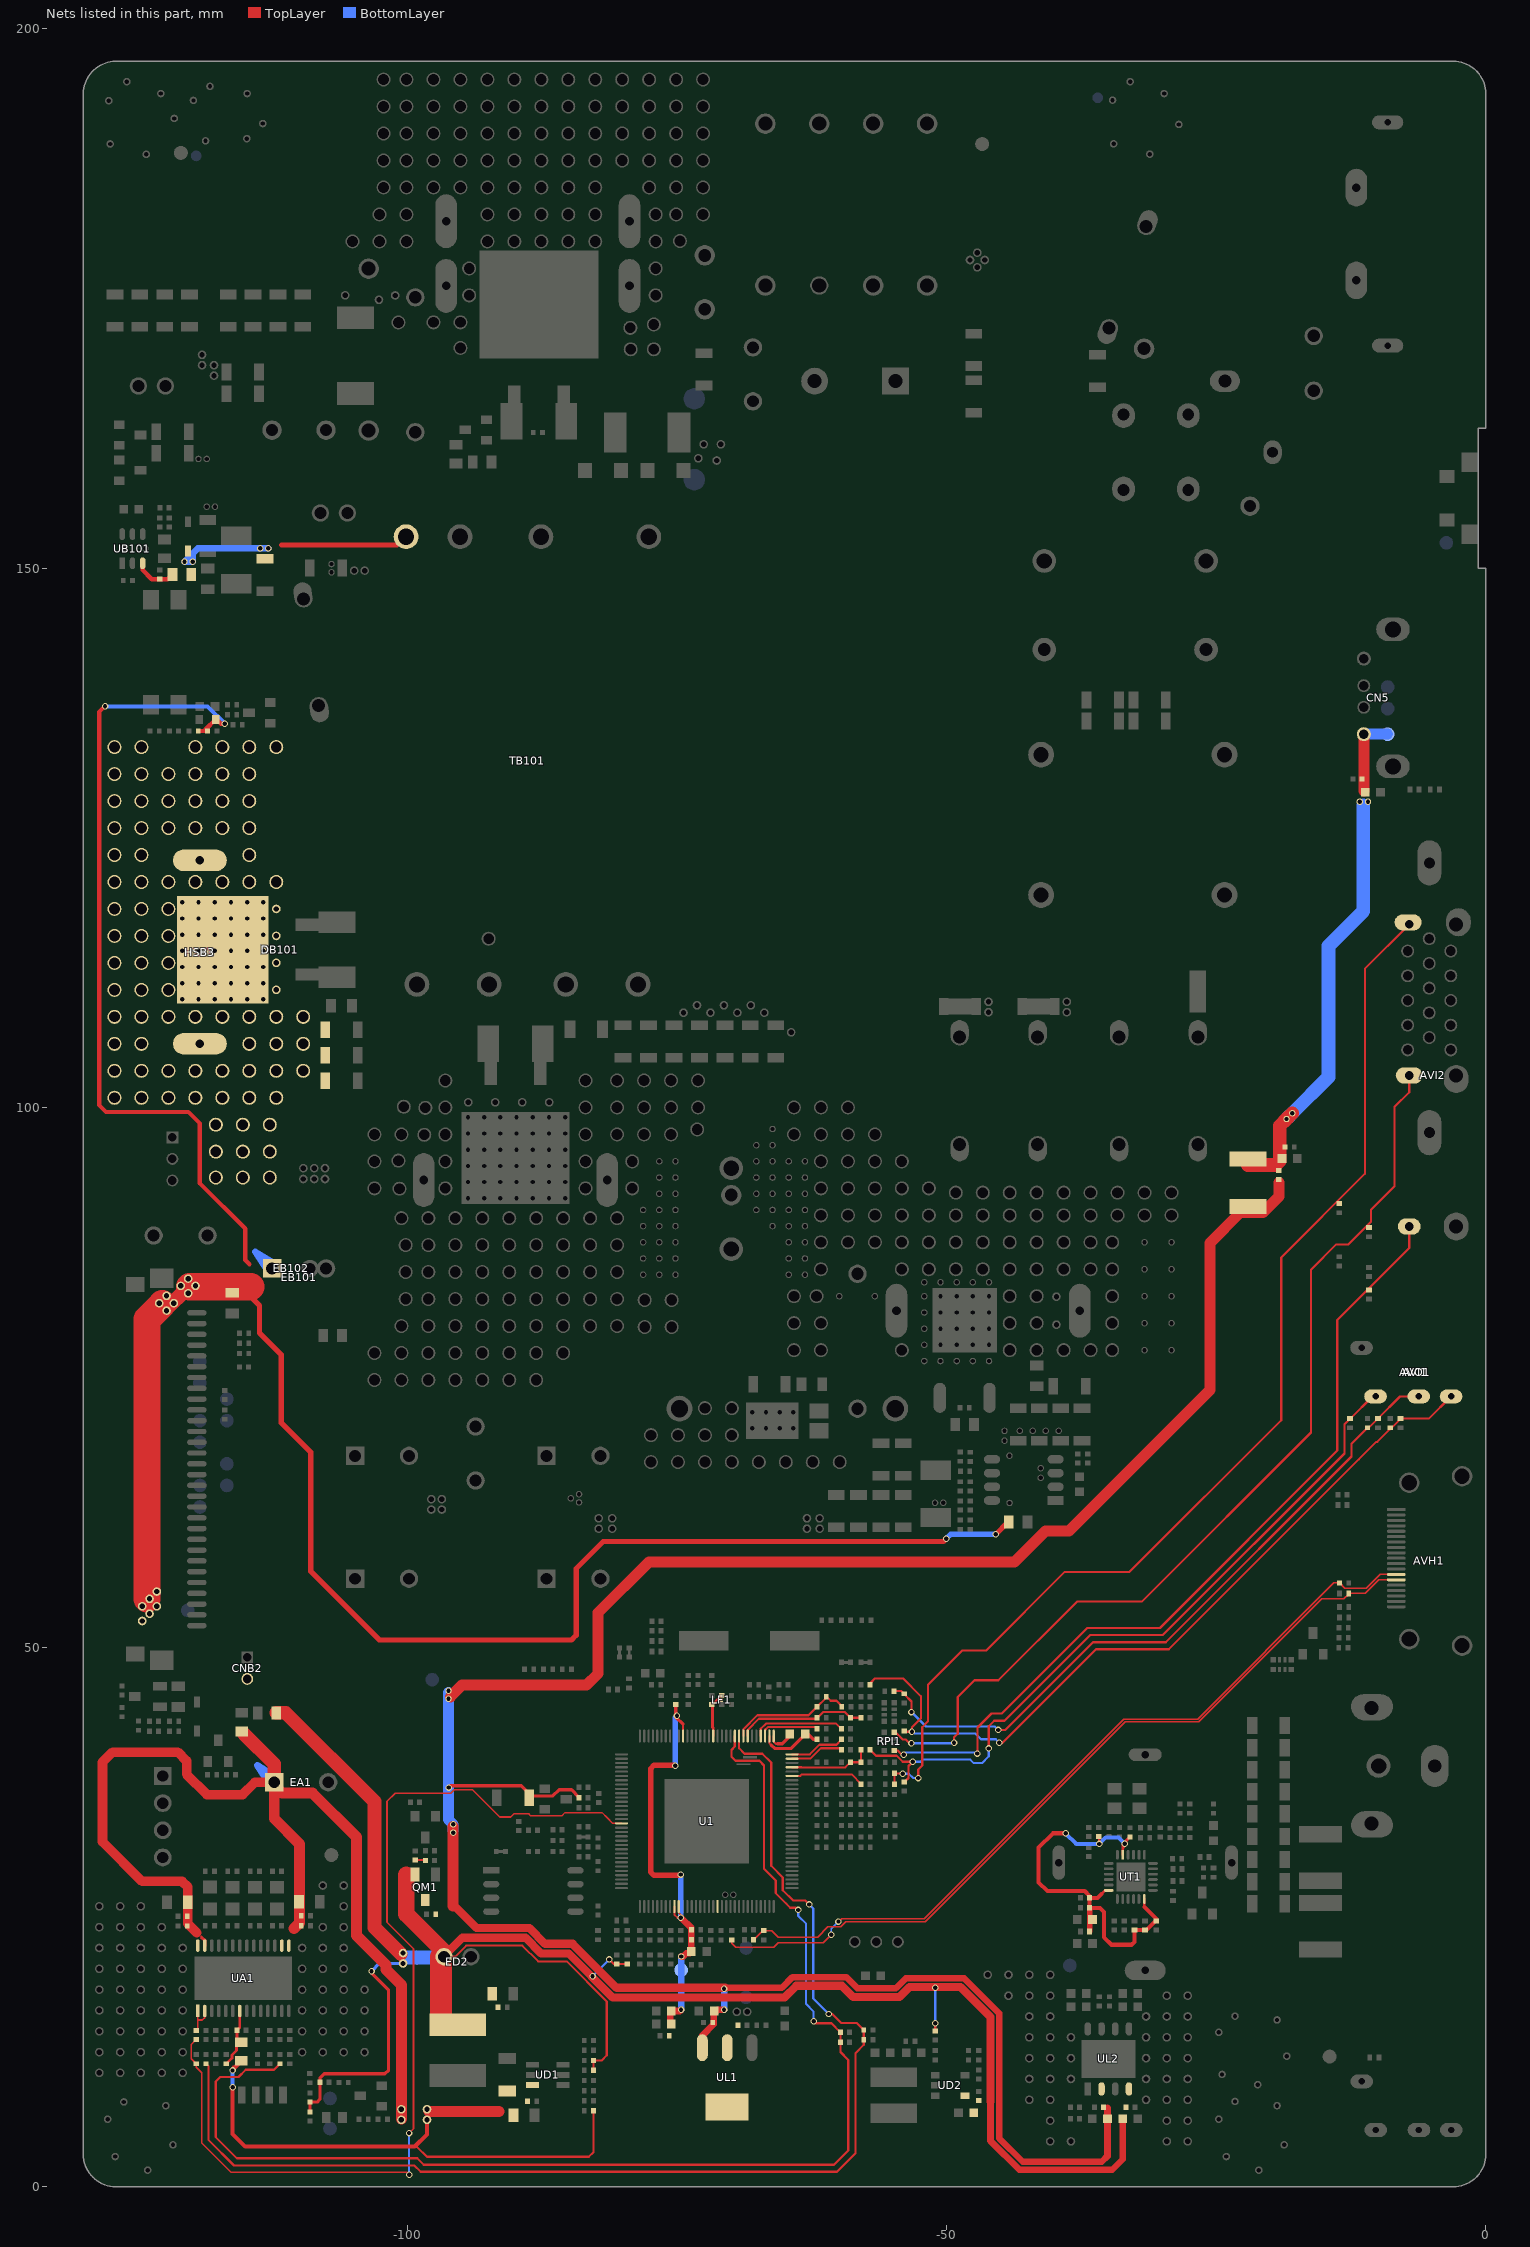
[diagram p0: the nets of this part, all layers, seen from the top]
# Altium PCB MISC84438.PcbDoc (part 7 of 15)
Units mm, origin at the board's own origin, x right, y up, seen from the top; angles counter-clockwise.
Board outline 130 x 197 mm, 2 copper layers (TopLayer, BottomLayer), stack 1.571 mm thick; 574 components, 314 nets, 2636 pads, 811 vias.

## Via types
v1: diameter 0.6, hole 0.4, TopLayer to BottomLayer, tented both sides, 780 vias
v2: diameter 0.7, hole 0.5, TopLayer to BottomLayer, tented both sides, 15 vias
v3: diameter 0.8, hole 0.6, TopLayer to BottomLayer, tented both sides, 12 vias
v4: diameter 0.8, hole 0.5, TopLayer to BottomLayer, tented both sides, 4 vias

## Nets (pads, with @x,y where several pads share a name; then routed paths per layer and width w, separated by ;. In a path a pad name is that pad's centre, name@x,y a point inside that pad or via, vN(x,y) a via of type N, cw(c..) or ccw(c..) an arc to the next point about the centre after c; other vN are vias at no path point) (continued)
3V3_Tun: CT5.2 CT6.1 CT9.1 CT18.2 CT27.1 LT1.1 LT2.2 LT12.2 RT18.1 UT1.11 UT1.18 UT1.24 | length 39
  TopLayer w0.203: RT18.1@-35.89,32.443 -35.839,32.392 v1(-35.839,31.763) ; UT1.11@-33.656,30.764 -33.656,31.407 -33.617,31.445
  TopLayer w0.229: -35.631,27.122 -35.29,27.464 UT1.18@-34.956,27.464 ; UT1.24@-31.656,26.664 -31.656,25.915 -31.648,25.908
  TopLayer w0.305: -33.617,31.445 -33.617,31.782 v1@-33.477,31.921 ; v1(-33.477,31.788) v1@-33.477,31.921 ; CT27.1@-32.982,32.417 v1@-33.477,31.921
  TopLayer w0.381: v1(-38.951,32.753) -40.132,32.753 -41.453,31.432 -41.453,28.194 -40.648,27.389 -37.179,27.389 -36.735,26.945 CT18.2@-36.735,26.772 ; -35.631,27.122 -35.982,26.772 CT18.2@-36.735,26.772 ; -31.648,25.908 -30.543,24.803 CT9.1@-30.543,24.631 -30.618,24.631 -31.468,23.781 LT1.1@-31.61,23.781 LT2.2@-32.575,23.781 -32.575,22.693 -32.848,22.42 -34.689,22.42 -35.382,23.114 -35.382,25.451 -35.776,25.844 CT5.2@-36.735,25.844 CT18.2@-36.735,26.772
  TopLayer w0.508: LT12.2@-36.735,23.66 CT5.2@-36.735,25.844
  BottomLayer w0.381: v1(-38.951,32.753) -37.96,31.763 v1(-35.839,31.763) -35.235,32.367 -34.057,32.367 v1(-33.477,31.788)
5V_M: CL1.2 CL2.2 CL6.2 CL7.2 CM2.1 F1.2 F2.1 pad.VIA5@-95.72,32.817 pad.VIA5@-95.72,33.579 pad.VIA5@-96.152,45.212 pad.VIA5@-96.152,45.974 QM1.D RO2.2 RO6.1 UL1.3 UL2.2 | length 232.1
  TopLayer w0.305: v1(-96.139,36.995) -95.987,37.147 -89.42,37.147 -88.493,36.22 -88.484,36.211 -86.471,36.211 -85.903,36.779 -84.75,36.779 -84.067,36.096 RO6.1@-84.067,36.065
  TopLayer w0.61: UL1.3@-72.623,12.877 -72.623,14.016 -71.577,15.062 -71.577,15.215 -71.577,16.002 -71.415,16.165 -71.183,16.396 v1(-70.612,16.396) ; v1@-70.51,18.433 -65.25,18.433 -64.255,19.428 -59.285,19.428 -58.253,18.396 -54.677,18.396 -53.75,19.323 -48.362,19.323 -45.098,16.058 -45.098,4.47 -42.926,2.299 -35.598,2.299 -35.07,2.827 CL7.2@-35.07,6.299 -35.07,7.29
  TopLayer w0.762: -95.606,26.01 -93.561,23.965 -88.648,23.965 -87.192,22.509 -84.64,22.509 -80.563,18.433 -70.612,18.433 v1@-70.51,18.433
  TopLayer w1.016: pad.VIA5@-95.987,45.402 -95.784,45.606 -94.907,46.482 -83.347,46.482 -82.283,47.546 -82.283,53.197 -77.568,57.912 -43.69,57.912 -40.819,60.782 -38.633,60.782 -25.578,73.838 -25.578,87.483 -22.76,90.301 -22.041,90.301 -20.66,90.301 -19.184,91.777 -19.184,93.098 ; -95.72,26.01 pad.VIA5@-95.72,32.817 pad.VIA5@-95.72,33.393
  BottomLayer w0.61: v1(-70.612,16.396) v1(-70.612,18.351)
  BottomLayer w1.016: pad.VIA5@-96.152,45.796 pad.VIA5@-96.152,45.212 -96.152,36.995 -96.152,34.011 pad.VIA5@-95.72,33.579 pad.VIA5@-95.72,33.033
5V_STB: 5V_STB.1 CD11.2 CD12.1 CD20.1 CD21.1 CD22.1 CL8.2 CL9.2 CM1.1 ED2.1 LD3.2 pad.VIA5@-100.368,20.688 pad.VIA5@-100.368,21.653 QM1.S R5V.1 RD8.1 RD13.2 RF8.2 RF9.2 RK1.2 RK13.1 RK15.1 RM1.2 UD2.4 UL2.4 | length 188.3
  TopLayer w0.203: RM1.2@-99.238,30.265 -98.323,30.265 CM1.1@-98.291,30.233 ; ED2.1@-96.846,21.311 ED2.1@-96.576,21.311 -95.53,21.311 -94.502,22.339 -89.306,22.339 -87.846,20.879 -85.204,20.879 -81.483,17.158 -81.483,12.167 -81.953,11.697 CD20.1@-82.721,11.697 RD13.2@-82.721,10.771 ; v1(-81.255,21.057) -80.827,20.629 RF8.2@-80.543,20.629 RF9.2@-79.578,20.629 ; RD8.1@-51.027,14.433 v1(-51.029,15.151)
  TopLayer w0.305: RK15.1@-108.991,6.927 RK13.1@-108.991,7.843 -108.324,7.843 -108.07,8.097 RK1.2@-108.07,9.677 -108.07,10.065 -107.675,10.461 -102.045,10.461 -101.711,10.795 -101.711,18.203 -103.289,19.781 v1(-103.289,19.977)
  TopLayer w0.61: -45.91,7.899 -45.91,4.242 -43.231,1.562 -34.633,1.562 -33.663,2.532 CL8.2@-33.663,6.299
  TopLayer w0.762: ED2.1@-96.139,21.806 -94.869,23.076 -89.016,23.076 -87.561,21.62 -85.008,21.62 -80.932,17.544 -64.99,17.544 -63.918,18.615 -59.673,18.615 -58.641,17.583 -54.341,17.583 -53.414,18.51 -48.699,18.51 -45.91,15.722 -45.91,7.899
  TopLayer w1.27: R5V.1@-112.113,43.917 -111.24,43.917 -103.022,35.699 -103.022,24.017 pad.VIA5@-100.568,21.562
  TopLayer w1.524: -100.051,28.905 -100.051,25.248 ED2.1@-96.576,21.773
  TopLayer w2.032: LD3.2@-96.846,15.164 ED2.1@-96.846,21.311
  BottomLayer w0.203: v1(-82.804,19.507) v1(-81.255,21.057) ; v1(-51.029,15.151) v1(-51.029,18.44)
  BottomLayer w0.305: v1(-103.289,19.977) -102.578,20.688 pad.VIA5@-100.368,20.688
  BottomLayer w1.27: -100.127,21.234 5V_STB.1@-99.085,21.234 -97.092,21.234 ED2.1@-96.576,21.234
5V_USB: CN5.1@-11.31,134.63 CU1.2 CU2.1 CU3.1 CU4.2 F1.1 F2.2 pad.VIA5@-10.922,128.372 pad.VIA5@-11.684,128.372 pad.VIA5@-17.936,99.502 pad.VIA5@-18.475,98.964 USB_5V.1 | length 47.2
  TopLayer w1.016: CU1.2@-11.31,129.375 -11.31,130.48 CN5.1@-11.31,134.63
  TopLayer w1.27: F1.1@-22.041,94.701 -19.472,94.701 -19.106,95.067 -19.106,95.301 -19.106,96.368 -19.106,98.333 pad.VIA5@-18.475,98.964 pad.VIA5@-17.936,99.502
  BottomLayer w1.016: CN5.1@-11.31,134.63 USB_5V.1@-9.096,134.63
  BottomLayer w1.27: pad.VIA5@-18.295,99.143 pad.VIA5@-17.936,99.502 -14.592,102.846 -14.592,115.008 -11.354,118.246 -11.354,128.016
12V: CA16.2 CA23.2 CA24.2 CA25.2 CA31.2 CA32.2 CB131.1 CD1.1 CD19.1 CD41.2 CNB2.2 DB101.2 EA1.1@-112.304,37.486 EB101.1@-112.5,85.114 EB102.1@-112.5,85.114 HSB3.1@-119.2,122.938 HSB3.2 pad.VIA5@-98.146,6.198 pad.VIA5@-98.146,7.163 pad.VIA5@-100.517,6.198 pad.VIA5@-100.517,7.163 pad.VIA5@-109.619,103.432 pad.VIA5@-109.619,105.932 pad.VIA5@-109.619,108.432 pad.VIA5@-112.119,100.932 pad.VIA5@-112.119,103.432 pad.VIA5@-112.119,105.932 pad.VIA5@-112.119,108.432 pad.VIA5@-112.119,110.932 pad.VIA5@-112.119,113.432 pad.VIA5@-112.119,115.932 pad.VIA5@-112.119,118.432 pad.VIA5@-112.119,120.932 pad.VIA5@-112.119,133.432 pad.VIA5@-112.719,93.532 pad.VIA5@-112.719,95.932 pad.VIA5@-112.719,98.432 pad.VIA5@-113.321,110.05 pad.VIA5@-113.321,111.55 pad.VIA5@-113.321,113.05 pad.VIA5@-113.321,114.55 pad.VIA5@-113.321,116.05 pad.VIA5@-113.321,117.55 pad.VIA5@-113.321,119.05 pad.VIA5@-114.619,100.932 pad.VIA5@-114.619,103.432 pad.VIA5@-114.619,105.932 pad.VIA5@-114.619,108.432 pad.VIA5@-114.619,120.932 pad.VIA5@-114.619,123.432 pad.VIA5@-114.619,125.932 pad.VIA5@-114.619,128.432 pad.VIA5@-114.619,130.932 pad.VIA5@-114.619,133.432 pad.VIA5@-114.821,110.05 pad.VIA5@-114.821,111.55 pad.VIA5@-114.821,113.05 pad.VIA5@-114.821,114.55 pad.VIA5@-114.821,116.05 pad.VIA5@-114.821,117.55 pad.VIA5@-114.821,119.05 pad.VIA5@-115.219,93.532 pad.VIA5@-115.219,95.932 pad.VIA5@-115.219,98.432 pad.VIA5@-116.321,110.05 pad.VIA5@-116.321,111.55 pad.VIA5@-116.321,113.05 pad.VIA5@-116.321,114.55 pad.VIA5@-116.321,116.05 pad.VIA5@-116.321,117.55 pad.VIA5@-116.321,119.05 pad.VIA5@-117.119,100.932 pad.VIA5@-117.119,103.432 pad.VIA5@-117.119,108.432 pad.VIA5@-117.119,120.932 pad.VIA5@-117.119,125.932 pad.VIA5@-117.119,128.432 pad.VIA5@-117.119,130.932 pad.VIA5@-117.119,133.432 pad.VIA5@-117.719,93.532 pad.VIA5@-117.719,95.932 pad.VIA5@-117.719,98.432 pad.VIA5@-117.821,110.05 pad.VIA5@-117.821,111.55 pad.VIA5@-117.821,113.05 pad.VIA5@-117.821,114.55 pad.VIA5@-117.821,116.05 pad.VIA5@-117.821,117.55 pad.VIA5@-117.821,119.05 pad.VIA5@-119.321,110.05 pad.VIA5@-119.321,111.55 pad.VIA5@-119.321,113.05 pad.VIA5@-119.321,114.55 pad.VIA5@-119.321,116.05 pad.VIA5@-119.321,117.55 pad.VIA5@-119.321,119.05 pad.VIA5@-119.607,83.49 pad.VIA5@-119.619,100.932 pad.VIA5@-119.619,103.432 pad.VIA5@-119.619,108.432 pad.VIA5@-119.619,120.932 pad.VIA5@-119.619,125.932 pad.VIA5@-119.619,128.432 pad.VIA5@-119.619,130.932 pad.VIA5@-119.619,133.432 pad.VIA5@-120.29,82.807 pad.VIA5@-120.29,84.172 pad.VIA5@-120.821,110.05 pad.VIA5@-120.821,111.55 pad.VIA5@-120.821,113.05 pad.VIA5@-120.821,114.55 pad.VIA5@-120.821,116.05 pad.VIA5@-120.821,117.55 pad.VIA5@-120.821,119.05 pad.VIA5@-120.972,83.49 pad.VIA5@-121.607,81.89 pad.VIA5@-122.29,81.207 pad.VIA5@-122.29,82.572 pad.VIA5@-122.119,100.932 pad.VIA5@-122.119,103.432 pad.VIA5@-122.119,108.432 pad.VIA5@-122.119,110.932 pad.VIA5@-122.119,113.432 pad.VIA5@-122.119,115.932 pad.VIA5@-122.119,118.432 pad.VIA5@-122.119,120.932 pad.VIA5@-122.119,125.932 pad.VIA5@-122.119,128.432 pad.VIA5@-122.119,130.932 pad.VIA5@-122.972,81.89 pad.VIA5@-123.182,53.797 pad.VIA5@-123.182,55.162 pad.VIA5@-123.865,53.115 pad.VIA5@-123.865,54.48 pad.VIA5@-124.547,52.432 pad.VIA5@-124.547,53.797 pad.VIA5@-124.619,100.932 pad.VIA5@-124.619,103.432 pad.VIA5@-124.619,105.932 pad.VIA5@-124.619,108.432 pad.VIA5@-124.619,110.932 pad.VIA5@-124.619,113.432 pad.VIA5@-124.619,115.932 pad.VIA5@-124.619,118.432 pad.VIA5@-124.619,120.932 pad.VIA5@-124.619,123.432 pad.VIA5@-124.619,125.932 pad.VIA5@-124.619,128.432 pad.VIA5@-124.619,130.932 pad.VIA5@-124.619,133.432 pad.VIA5@-127.119,100.932 pad.VIA5@-127.119,103.432 pad.VIA5@-127.119,105.932 pad.VIA5@-127.119,108.432 pad.VIA5@-127.119,110.932 pad.VIA5@-127.119,113.432 pad.VIA5@-127.119,115.932 pad.VIA5@-127.119,118.432 pad.VIA5@-127.119,120.932 pad.VIA5@-127.119,123.432 pad.VIA5@-127.119,125.932 pad.VIA5@-127.119,128.432 pad.VIA5@-127.119,130.932 pad.VIA5@-127.119,133.432 R12V.1 RA3.1 RB128.2 RB129.2 RB131.2 RB135.1 RB158.2 RB165.2 RB816.1 RD14.1 UA1.15 UA1.16 UA1.27 UA1.28 UD1.3 | length 371.2
  TopLayer w0.203: -99.083,3.711 -98.141,2.769 -83.147,2.769 -82.721,3.195 RD14.1@-82.721,7.048
  TopLayer w0.305: -119.055,23.134 -118.75,22.828 UA1.27@-118.75,22.34
  TopLayer w0.381: v1(-116.167,9.22) -116.167,4.877 -114.998,3.708 -99.284,3.708 -98.146,4.847 pad.VIA5@-98.146,6.198 ; v1@-116.093,11.024 v1@-116.093,10.93 ; RA3.1@-115.367,11.656 v1@-116.093,10.93 ; v1@-116.093,10.93 -116.174,10.849 v1(-116.174,10.773) -116.093,10.854 v1@-116.093,10.93
  TopLayer w0.4: v1(-127.991,137.236) -128.537,136.69 -128.537,100.256 -127.9,99.619 -120.266,99.619 -119.197,98.55 -119.197,92.997 -115,88.8 -115,85.9 -114.6,85.5 ; RB158.2@-119.356,134.925 -118.814,134.925 RB135.1@-118.646,135.093 ; RB135.1@-118.479,134.925 RB135.1@-118.646,135.093 ; RB131.2@-117.735,136.004 RB131.2@-117.747,135.992 ; v1(-116.9,135.6) -117.241,135.6 -117.633,135.992 RB131.2@-117.747,135.992 ; RB135.1@-118.646,135.093 RB131.2@-117.747,135.992
  TopLayer w0.5: -114.5,82.5 -113.678,81.678 -113.678,79.132 -111.651,77.104 -111.651,70.798 -108.912,68.06 -108.912,57.018 -102.563,50.669 -84.766,50.669 -84.311,51.124 -84.311,57.296 -81.81,59.798 -50.286,59.798 v1(-50.025,60.058) ; v1(-45.426,60.463) RB816.1@-44.294,61.595
  TopLayer w0.889: CA31.2@-120.319,26.365 -120.319,27.774 -120.845,28.3 -124.553,28.3 -128.222,31.969 -128.222,39.342 -127.284,40.28 -121.237,40.28 -120.426,39.469 -120.426,38.22 -118.541,36.335 -115.24,36.335 -114.088,37.486 EA1.1@-112.304,37.486 ; CA31.2@-120.308,26.365 -120.308,24.355 -119.499,23.546
  TopLayer w1.016: -110.464,23.913 -109.953,24.424 -109.953,31.759 -112.304,34.11 -112.304,37.207 -111.572,36.474 -108.779,36.474 -104.699,32.394 -104.699,23.291 -101.943,20.535 -101.943,20.123 -100.517,18.697 pad.VIA5@-100.517,7.163 pad.VIA5@-100.517,6.274 ; pad.VIA5@-97.98,6.972 -91.453,6.972
  TopLayer w1.27: R12V.1@-115.101,41.972 -112.304,39.175 EA1.1@-112.304,37.486
  TopLayer w1.346: pad.VIA5@-122.204,81.458 -120.573,83.09 -120.258,83.404 -120.163,83.404
  TopLayer w2.54: pad.VIA5@-124.097,54.508 -124.097,80.41 -122.795,81.712 pad.VIA5@-122.68,81.827 ; -120.163,83.404 -114.496,83.404
  BottomLayer w0.381: v1(-116.174,10.773) -116.174,9.227 v1(-116.167,9.22)
  BottomLayer w0.4: v1(-127.991,137.236) -127.948,137.193 -118.493,137.193 v1(-116.9,135.6)
  BottomLayer w0.5: v1(-50.025,60.058) -49.621,60.463 v1(-45.426,60.463)
12V-OVP: DB112.A pad.VIA5@-112.852,151.854 pad.VIA5@-113.614,151.854 pad.VIA5@-119.863,150.628 pad.VIA5@-120.625,150.628 RB113.2 RB114.2 TB101.5 | length 20.5
  TopLayer w0.5: -111.63,152.17 -100.958,152.17
  BottomLayer w0.6: pad.VIA5@-112.852,151.854 pad.VIA5@-113.614,151.854 -119.399,151.854 -119.863,151.39 ; -119.863,151.39 pad.VIA5@-119.863,150.628 pad.VIA5@-120.625,150.628 -119.863,151.39
+1.8V_DDR: 1.8V_DDR.1 CF22.1 CF23.2 CF24.2 CF25.2 CL3.2 CL4.2 CL5.2 RL1.1 U1.54 U1.105 U1.106 UL1.2 UL1.4 | length 40.7
  TopLayer w0.178: U1.105@-75.212,25.971 -75.212,25.21 -74.917,24.915 v1(-74.612,24.915) ; U1.106@-74.812,25.971 -74.812,25.368 v1@-74.549,25.105 ; U1.54@-74.412,41.771 -74.412,42.739
  TopLayer w0.305: v1@-75.082,43.518 -74.412,42.847 ; v1@-75.082,43.634 CF23.2@-75.082,44.685
  TopLayer w0.508: v1@-75.184,39.065 -77.089,39.065 -77.42,38.734 -77.42,29.182 -77.094,28.857 v1@-74.612,28.857
  TopLayer w0.61: CL5.2@-75.598,15.07 -75.598,16.281 CL4.2@-75.497,16.281 -74.701,16.281 v1(-74.6,16.383) ; v1(-74.587,21.333) -74.416,21.333 -74.118,21.631 -73.801,21.631 CF22.1@-73.642,21.79 ; v1@-74.58,24.915 -73.642,23.977 CF22.1@-73.642,21.79 ; CF22.1@-73.642,21.671 CF22.1@-73.642,21.79
  BottomLayer w0.508: v1@-75.138,39.019 v1@-75.138,43.477 ; v1(-74.612,24.915) v1(-74.612,28.928)
  BottomLayer w0.61: v1(-74.6,16.383) -74.587,16.396 1.8V_DDR.1@-74.587,20.066 v1(-74.587,21.333)
  other v1: -75.133,39.014 -74.981,43.634
AMP-OUTL: CF29.1 RA21.1 RF14.2 U1.41 | length 115.6
  TopLayer w0.203: RA21.1@-118.629,11.397 -118.389,11.157 -118.389,4.314 -116.044,1.969 -99.317,1.969 -98.72,1.372 -60.143,1.372 -58.433,3.082 -58.433,12.373 -57.658,13.147 RF14.2@-57.658,13.602 CF29.1@-57.658,14.516 ; U1.41@-69.212,41.771 -69.212,40.626 -68.718,40.132 -67.061,40.132 -66.243,39.314 -66.243,29.733 -65.162,28.652 -65.162,27.482 -64.195,26.515 -63.081,26.515 v1(-62.725,26.159) ; v1(-60.909,16.002) -60.579,16.002 -59.747,15.17 -58.312,15.17 CF29.1@-57.658,14.516 ; CF29.1@-57.696,14.478 CF29.1@-57.658,14.516
  BottomLayer w0.203: v1(-62.725,26.159) -62.345,25.779 -62.345,17.438 v1(-60.909,16.002)
AMP-OUTR: CF30.1 RA5.1 RF15.2 U1.42 | length 117.6
  TopLayer w0.203: RA5.1@-111.772,11.397 -112.335,10.833 -114.957,10.833 -115.622,10.169 -117.314,10.169 -117.729,9.754 -117.729,7.899 -117.729,4.588 -115.77,2.629 -99.043,2.629 -98.446,2.032 -60.417,2.032 -59.093,3.356 -59.093,11.747 -59.822,12.476 -59.822,13.391 CF30.1@-59.83,13.399 RF15.2@-59.83,14.313 -60.66,15.143 -62.133,15.143 v1(-62.306,15.316) ; U1.42@-69.612,41.771 -69.612,40.791 -69.927,40.476 -69.927,39.845 -69.553,39.471 -67.335,39.471 -66.904,39.04 -66.904,29.46 -65.823,28.379 -65.823,27.209 -64.835,26.221 -64.468,25.854 -63.932,25.854 v1(-63.729,25.651)
  BottomLayer w0.203: v1(-63.729,25.651) -63.729,25.082 -63.006,24.36 -63.006,16.921 -62.308,16.223 -62.308,15.318 v1(-62.306,15.316)
AMP_STB: RA1.2 RA8.1 U1.81 | length 90.4
  TopLayer w0.152: RA8.1@-119.544,13.632 -119.997,13.179 -119.997,11.85 RA1.2@-119.544,11.397 -119.544,11.074 -119.024,10.554 -119.024,4.051 -116.307,1.334 -100.025,1.334 v1(-99.797,1.105) ; v1(-99.809,4.966) -99.399,5.376 -99.399,22.046 -101.854,24.501 -101.854,35.712 -101.092,36.474 -95.948,36.474 -95.631,36.792 -93.931,36.792 -91.404,34.265 -90.381,34.265 -90.086,34.559 -88.724,34.559 -88.548,34.382 -85.636,34.382 -85.346,34.672 -81.931,34.672 -81.451,34.192 -80.943,33.685 -80.126,33.685 U1.81@-80.112,33.671
  BottomLayer w0.152: v1(-99.809,4.966) -99.809,1.118 v1(-99.797,1.105)
AMP_STB/: RA8.2 UA1.1 UA1.2 | length 3.2
  TopLayer w0.152: RA8.2@-119.544,14.482 -119.4,14.626 -119.4,15.443 ; UA1.1@-119.4,16.29 -119.4,15.443 ; UA1.2@-118.75,16.29 -118.75,15.667 -118.974,15.443 -119.4,15.443
ARC: AVH1.14 CH15.1 DH3.K RH2.1 | length 73.9
  TopLayer w0.127: CH15.1@-67.876,22.872 -67.021,23.727 RH2.1@-66.916,23.727 -66.171,23.727 -65.569,23.124 -61.945,23.124 -60.986,24.083 -59.801,24.083 -59.328,24.556 -51.957,24.556 -48.099,28.414 -33.435,43.078 -26.619,43.078 -16.798,52.9 -15.206,54.492 -13.147,54.492 -12.707,54.932 DH3.K@-12.707,54.991 -11.19,54.991 -9.931,56.25 AVH1.14@-8.3,56.25
AUVAG: CF28.2 U1.33 | length 2.4
  TopLayer w0.203: U1.33@-66.012,41.771 -66.012,41.251 -65.808,41.046 -65.634,41.046
  TopLayer w0.305: -65.634,41.046 -65.227,41.046 CF28.2@-64.516,41.757
AUVRM: CF28.1 LF6.2 U1.34 | length 6.1
  TopLayer w0.203: U1.34@-66.412,41.771 -66.412,41.112 -66.231,40.931
  TopLayer w0.305: -66.231,40.931 -65.915,40.614 -64.394,40.614 -63.048,41.961 -62.865,41.961 -62.357,41.453 LF6.2@-61.995,41.453
AV1_LIN: CI7.1 U1.32 | length 5.2
  TopLayer w0.198: U1.32@-64.312,40.071 -62.672,40.071 -61.776,40.967 -60.189,40.967 -59.734,41.422 CI7.1@-59.734,41.452
AV1_RIN: CI6.1 U1.31 | length 5
  TopLayer w0.198: U1.31@-64.312,39.671 -62.612,39.671 -61.641,40.642 -59.876,40.642 CI6.1@-59.734,40.5
AV2_LIN: CI4.1 U1.36 | length 8.6
  TopLayer w0.198: U1.36@-67.212,41.771 -67.212,42.439 -66.73,42.922 -60.225,42.922 CI4.1@-59.734,42.431
AV2_RIN: CI3.1 U1.35 | length 5.6
  TopLayer w0.198: U1.35@-66.812,41.771 -66.812,42.332 -66.548,42.597 -62.161,42.597 CI3.1@-61.995,42.431
AV-OUTL: CO3.2 RO1.1 RO4.2 U1.39 | length 12
  TopLayer w0.203: U1.39@-68.412,41.771 -68.412,42.336 -67.384,43.364 -62.09,43.364 CO3.2@-61.995,43.459 -61.943,43.459 -61.414,43.988 -59.413,43.988 RO4.2@-58.884,43.459 RO1.1@-57.931,43.459
AV-OUTR: CO5.2 RO5.1 RO8.2 U1.40 | length 11.6
  TopLayer w0.203: U1.40@-68.812,41.771 -68.812,42.403 -67.521,43.694 -62.776,43.694 CO5.2@-61.995,44.475 ; CO5.2@-61.943,44.475 CO5.2@-61.995,44.475 ; RO5.1@-59.709,44.475 -59.709,44.561 -60.192,45.045 -60.723,45.045 -61.145,45.466 RO8.2@-61.145,45.416 -61.145,45.325 CO5.2@-61.995,44.475
AV_IN: CI8.1 U1.27 | length 6.9
  TopLayer w0.198: U1.27@-64.312,38.071 -63.551,38.071 -63.411,38.211 -58.778,38.211 CI8.1@-57.88,37.313
AV_L: AVI2.3 DI2.K RPI1.2 | length 90.6
  TopLayer w0.203: RPI1.2@-54.846,42.125 -54.723,42.125 -54.071,41.473 ; -54.046,41.461 -53.789,41.461 v1@-53.429,41.1 ; v1(-49.289,41.135) -49.311,41.158 -49.311,41.628 -48.952,41.987 -48.952,45.381 -47.4,46.933 -45.189,46.933 -37.893,54.229 -31.882,54.229 -16.205,69.905 -16.205,84.993 -13.855,87.343 -12.738,87.343 -10.643,89.438 -10.643,90.555 -8.458,92.74 -8.458,100.086 -7.1,101.444 AVI2.3@-7.1,103
  BottomLayer w0.203: v1(-53.243,41.1) -49.324,41.1 v1(-49.289,41.135)
AV_LIN/OUT: AVI1.4 AVO1.4 CI10.1 DO1.K RI13.1 RO13.1 | length 64.3
  TopLayer w0.203: RO13.1@-54.871,45.936 -54.199,45.936 RI13.1@-53.899,45.635 ; RI13.1@-53.899,45.687 RI13.1@-53.899,45.635 ; v1(-53.238,43.993) -53.238,44.975 RI13.1@-53.899,45.635 ; v1(-45.203,42.332) -44.546,42.332 -36.408,50.47 -29.661,50.47 -12.446,67.685 -12.446,68.866 CI10.1@-10.973,70.339 -10.858,70.339 DO1.K@-10.008,71.189 -7.947,73.25 AVO1.4@-6.222,73.25
  BottomLayer w0.203: v1(-53.238,43.993) -51.9,42.654 -45.525,42.654 v1(-45.203,42.332)
AV_R: AVI2.1 DI1.K RPI1.8 | length 77.9
  TopLayer w0.203: RPI1.8@-54.846,40.425 -54.522,40.425 -54.14,40.043 v1(-53.962,40.043) ; v1(-47.135,40.141) -47.123,40.153 -47.123,42.56 -45.817,43.866 -44.88,43.866 -36.955,51.791 -30.208,51.791 -13.767,68.232 -13.767,80.34 -7.1,87.007 AVI2.1@-7.1,89
  BottomLayer w0.203: v1(-53.962,40.043) -53.764,40.241 -47.236,40.241 v1(-47.135,40.141)
AV_RIN/ROUT: AVI1.3 AVO1.3 CI11.1 DO3.K RI15.1 RO15.1 | length 73.9
  TopLayer w0.203: RO15.1@-57.081,46.507 -57.081,46.643 -56.613,47.111 -54.029,47.111 -52.368,45.45 -52.368,43.402 -53.196,42.574 v1(-53.196,42.157) -53.809,42.157 RI15.1@-53.899,42.247 ; v1(-45.098,41.135) v1@-44.807,41.135 ; v1@-44.841,41.101 v1@-44.807,41.135 ; AVO1.3@-3.222,73.25 -5.282,71.189 DO3.K@-7.899,71.189 -10.052,69.037 -10.16,69.037 -11.786,67.412 -29.388,49.809 -36.133,49.809 v1@-44.807,41.135
  BottomLayer w0.203: v1(-53.196,42.157) -53.086,42.157 -52.922,41.994 -47.31,41.994 -46.79,41.473 -45.436,41.473 v1(-45.098,41.135)
AVCC: CA28.2 RA3.2 RA4.2 UA1.7 | length 5.4
  TopLayer w0.254: RA4.2@-116.737,11.397 -116.221,11.913 -116.221,12.211 -115.799,12.634 -115.799,13.284 -115.695,13.388 RA3.2@-115.367,13.388 ; RA3.2@-115.766,13.788 CA28.2@-115.766,14.503 -115.5,14.77 UA1.7@-115.5,16.29
AVDD5V_MHL: U1.115
AVDD_DMPLL: CF12.2 LF1.2 LF1.3 U1.47 | length 4.2
  TopLayer w0.203: U1.47@-71.612,41.771 -71.612,42.504
  TopLayer w0.254: -71.612,42.504 -71.679,42.57 -71.679,42.974 -71.676,42.977 -71.676,44.606 CF12.2@-71.755,44.685 -71.691,44.685 -71.053,45.323 LF1.2@-70.841,45.535
BRO: RB104.2 RB113.1 UB101.3 | length 3.9
  TopLayer w0.4: UB101.3@-124.5,150.477 -124.5,149.849 -123.654,149.003 RB104.2@-122.936,149.003 -122.17,149.003 RB113.1@-121.745,149.428
CEC: AVH1.13 CH10.2 RH13.1 | length 77.2
  TopLayer w0.127: RH13.1@-69.913,22.877 -69.913,22.543 -69.549,22.178 -66.013,22.178 -65.575,22.616 -61.4,22.616 v1(-60.678,23.338) ; v1(-60.005,24.573) -59.927,24.573 -59.691,24.81 -52.063,24.81 -48.279,28.594 -33.54,43.332 -26.724,43.332 -14.101,55.956 CH10.2@-13.593,55.956 ; CH10.2@-13.557,55.992 CH10.2@-13.593,55.956 ; AVH1.13@-8.3,56.75 -9.79,56.75 -11.084,55.456 -13.057,55.456 CH10.2@-13.557,55.956 CH10.2@-13.593,55.956
  BottomLayer w0.127: v1(-60.678,23.338) -60.678,23.9 v1(-60.005,24.573)
CVBS_IN: AVI2.5 DI3.K RI8.1 RI9.2 | length 106.2
  TopLayer w0.203: RI8.1@-54.82,37.313 RI9.2@-54.82,38.303 -54.077,38.303 v1(-54.051,38.278) ; v1(-52.603,37.871) -52.603,38.674 -52.248,39.03 -52.248,42.589 -51.708,43.129 -51.708,46.522 -48.529,49.701 -46.318,49.701 -39.035,56.985 -38.557,56.985 -33.023,56.985 -18.961,71.047 -18.961,86.134 -11.214,93.881 -11.214,112.886 AVI2.5@-7.1,117
  BottomLayer w0.203: v1@-54.013,38.316 v1(-54.051,38.278) -53.479,38.278 -53.073,37.871 v1(-52.603,37.871)
CVBS_IN/OUT: AVI1.2 AVO1.2 DO2.K RI14.1 RO14.1 | length 67
  TopLayer w0.203: RO14.1@-57.081,40.5 -56.526,39.946 -54.615,39.946 -54.051,39.383 v1(-53.124,39.383) -53.523,38.984 -53.523,37.885 RI14.1@-53.899,37.509 ; v1(-46.076,40.615) -46.076,42.674 -45.558,43.191 -44.621,43.191 -36.682,51.13 -29.935,51.13 -13.106,67.959 -13.106,70.656 DO2.K@-12.573,71.189 -10.512,73.25 AVO1.2@-10.222,73.25
  BottomLayer w0.203: v1(-53.124,39.383) -52.421,39.383 -52.222,39.581 -47.79,39.581 -47.465,39.256 -46.711,39.256 -46.076,39.891 v1(-46.076,40.615)
CVBS_OUT: CO9.2 RO12.1 RO14.2 U1.29 | length 7.7
  TopLayer w0.198: U1.29@-64.312,38.871 -63.431,38.871 -63.421,38.861 -59.367,38.861 RO12.1@-58.884,39.344 CO9.2@-57.931,39.344 RO14.2@-57.931,40.5